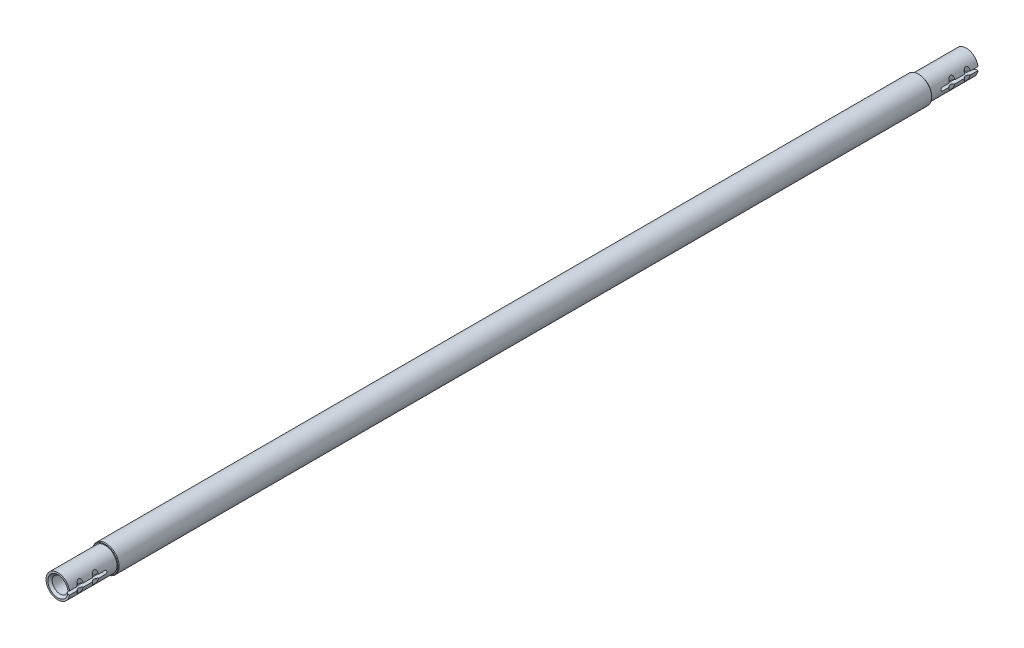
SolidWorks part; units mm, degrees
material "普通碳钢"
ref_plane "前视基准面" through (0, 0, 0) normal (0, 0, 1) x (1, 0, 0)
ref_plane "上视基准面" through (0, 0, 0) normal (0, 1, 0) x (1, 0, 0)
ref_plane "右视基准面" through (0, 0, 0) normal (1, 0, 0) x (0, 0, -1)
sketch "草图2" plane through (0, 0, 0) normal (0, 0, 1) x (1, 0, 0)
  circle A0 centre (0, 0) radius 22.5
  dimension "D1" = 45
extrude "凸台-拉伸1" add sketch "草图2" along normal mid plane 1535
sketch "草图3" plane through (0, 0, 767.5) normal (0, 0, 1) x (1, 0, 0)
  circle A0 centre (0, 0) radius 22.5 construction
  circle A1 centre (0, 0) radius 22.5
  circle A2 centre (0, 0) radius 20
  dimension "D1" = 40
extrude "切除-拉伸1" cut sketch "草图3" against normal blind 80
ref_plane "基准面1" through (0, 0, 667.5) normal (0, 0, 1) x (1, 0, 0)
sketch "草图4" plane through (0, 0, 667.5) normal (0, 0, 1) x (1, 0, 0)
  circle A0 centre (0, 0) radius 16
  dimension "D1" = 32
extrude "切除-拉伸2" cut sketch "草图4" along normal blind 30
mirror "镜向1" about plane through (0, 0, 0) normal (0, 0, 1) of "切除-拉伸2", "切除-拉伸1"
sketch "草图5" plane through (0, 0, 667.5) normal (0, 0, 1) x (1, 0, 0)
  circle A0 centre (0, 0) radius 12.5
  dimension "D1" = 25
extrude "切除-拉伸3" cut sketch "草图5" against normal up to next
hole_wizard "M30 螺纹孔1" positions "草图7" profile "草图6" tap size "M30" standard "GB"
sketch "草图7" plane through (0, 0, 767.5) normal (0, 0, 1) x (1, 0, 0)
  point P0 (0, 0)
sketch "草图6" plane through (0, 0, 767.5) normal (1, 0, 0) x (0, -1, 0)
  line L0 (0, 0) -> (0, 70)
  line L1 (0, 70) -> (13.25, 70)
  line L2 (13.25, 70) -> (13.25, 3.75)
  line L3 (13.25, 3.75) -> (17, 0)
  line L5 (17, 0) -> (0, 0)
  line L6 (-13.25, 3.75) -> (-17, 0) construction
  line L11 (0, -6.35) -> (0, 107.95) construction
  dimension "通孔螺纹孔钻头直径" = 26.5
  dimension "通孔螺纹孔钻头深度" = 70
  dimension "近端锥形沉头孔直径" = 34
  dimension "近端锥形沉头孔角度" = 90
cosmetic thread "孔螺蚊线1" parameters "D2"=30
hole_wizard "M30 螺纹孔2-左旋" positions "草图9" profile "草图8" tap size "M30" standard "GB"
sketch "草图9" plane through (0, 0, -767.5) normal (0, 0, -1) x (-1, 0, 0)
  point P0 (0, 0)
sketch "草图8" plane through (0, 0, -767.5) normal (1, 0, 0) x (0, 1, 0)
  line L0 (0, 0) -> (0, 70)
  line L1 (0, 70) -> (13.25, 70)
  line L2 (13.25, 70) -> (13.25, 3.75)
  line L3 (13.25, 3.75) -> (17, 0)
  line L5 (17, 0) -> (0, 0)
  line L6 (-13.25, 3.75) -> (-17, 0) construction
  line L11 (0, -6.35) -> (0, 107.95) construction
  dimension "通孔螺纹孔钻头直径" = 26.5
  dimension "通孔螺纹孔钻头深度" = 70
  dimension "近端锥形沉头孔直径" = 34
  dimension "近端锥形沉头孔角度" = 90
cosmetic thread "孔螺蚊线2" parameters "D2"=30
sketch "草图10" plane through (0, 0, 0) normal (0, 1, 0) x (1, 0, 0)
  line L0 (-623.6737, 0) -> (575.7315, 0) construction
  line L1 (0, 878.5975) -> (0, -1113.4942) construction
  line L2 (23, 878.5975) -> (23, -1113.4942) construction
  line L3 (-20, -767.5) -> (20, -767.5) construction
  line L4 (-20, -767.5) -> (20, -767.5) construction
  circle A0 centre (23, -749.5) radius 6
  circle A1 centre (23, -723.5) radius 6
  dimension "D4" = 12
  dimension "D1" = 23
  dimension "D2" = 18
  dimension "D3" = 26
extrude "切除-拉伸4" cut sketch "草图10" against normal through all both and the other way through all
sketch "草图11" plane through (0, 0, 0) normal (1, 0, 0) x (0, 0, -1)
  line L0 (-870.3922, 0) -> (-91.3244, 0) construction
  line L1 (-767.5, 20) -> (-767.5, -20) construction
  line L2 (-767.5, 20) -> (-767.5, -20) construction
  line L3 (-767.5, 0) -> (-707.5, 0) construction
  line L4 (-767.5, 3) -> (-707.5, 3)
  line L5 (-767.5, -3) -> (-707.5, -3)
  arc A0 (-767.5, 3) -> (-767.5, -3) centre (-767.5, 0) ccw
  arc A1 (-707.5, -3) -> (-707.5, 3) centre (-707.5, 0) ccw
  point P9 (-737.5, 0)
  dimension "D1" = 6
  dimension "D2" = 60
extrude "切除-拉伸5" cut sketch "草图11" along normal through all
mirror "镜向2" about plane through (0, 0, 0) normal (0, 0, 1) of "切除-拉伸5", "切除-拉伸4"
chamfer "倒角1" distance 1 angle 45 2 edges at (22.5, 0, -687.5) (22.5, 0, 687.5)
